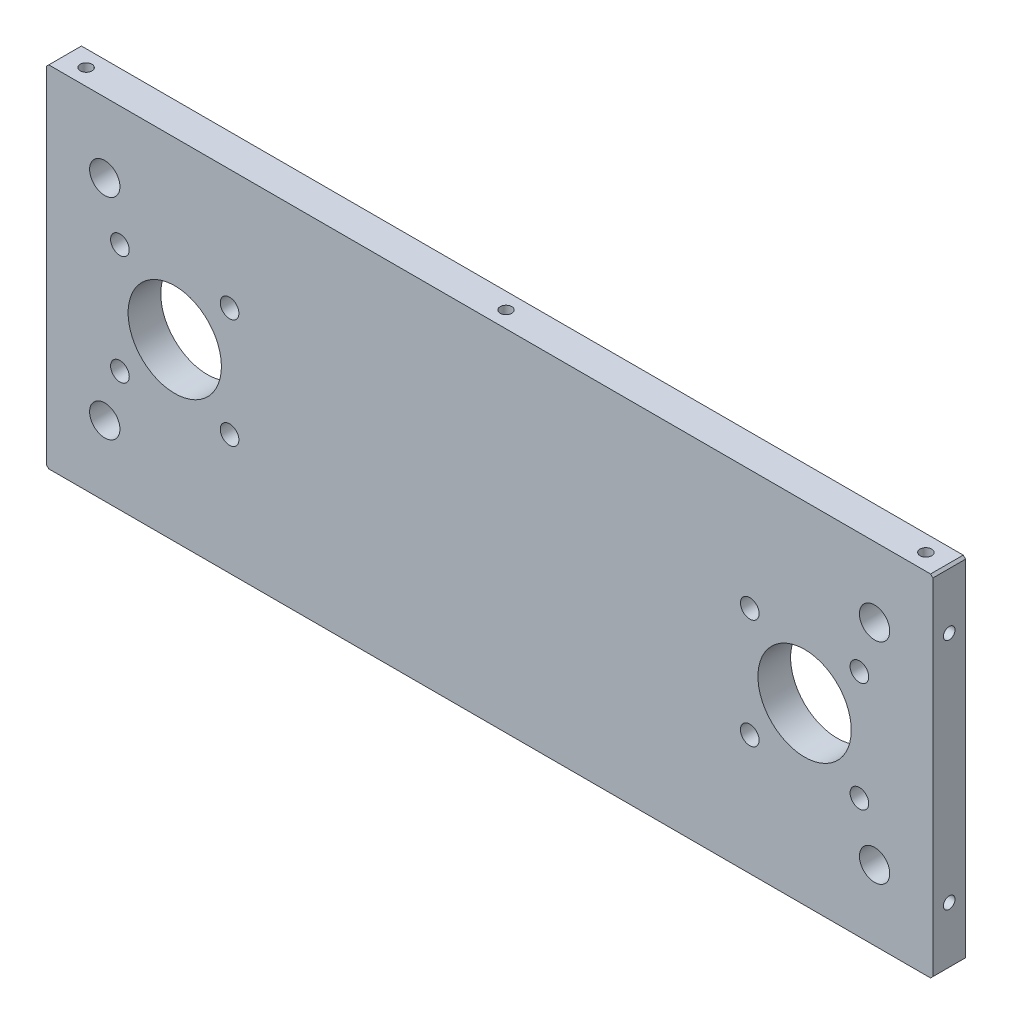
from build123d import *

# Parameters (mm, degrees)
SKETCH1_W                  = 380
SKETCH1_H                  = 150
BOSS_EXTRUDE1_DEPTH        = 14
CHAMFER1_SIZE              = 1
SKETCH2_R                  = 20
CUT_EXTRUDE1_DEPTH         = 409.773776067
F_8_0_8_DIAMETER_HOLE1_D   = 8
LPATTERN1_COUNT            = 2
LPATTERN1_PITCH            = 270
F_13_0_13_DIAMETER_HOLE1_D = 13
M6_TAPPED_HOLE1_D          = 5
M6_TAPPED_HOLE1_DEPTH      = 15
M6_TAPPED_HOLE1_TIP        = 1.502151548
M6_TAPPED_HOLE2_D          = 5
M6_TAPPED_HOLE2_DEPTH      = 15
M6_TAPPED_HOLE2_TIP        = 1.502151548
M6_TAPPED_HOLE3_D          = 5
M6_TAPPED_HOLE3_DEPTH      = 15
M6_TAPPED_HOLE3_TIP        = 1.502151548
M6_TAPPED_HOLE4_D          = 5
M6_TAPPED_HOLE4_DEPTH      = 15
M6_TAPPED_HOLE4_TIP        = 1.502151548


with BuildPart() as part:
    # Sketch1 → Boss-Extrude1 (new body)
    with BuildSketch(Plane.XY):
        with Locations((190, 75)):
            Rectangle(SKETCH1_W, SKETCH1_H)
    extrude(amount=BOSS_EXTRUDE1_DEPTH)

    # Chamfer1
    chamfer1_edges = [part.edges().sort_by_distance(p)[0] for p in [
        (0, 150, 7),
        (380, 150, 7),
        (380, 0, 7),
        (0, 0, 7),
    ]]
    chamfer(chamfer1_edges, length=CHAMFER1_SIZE)

    # Sketch2 → Cut-Extrude1 (cut, through all)
    with BuildSketch(Plane.XY.offset(14)):
        with Locations((55, 75)):
            Circle(SKETCH2_R)
        with Locations((325, 75)):
            Circle(SKETCH2_R)
    extrude(amount=-CUT_EXTRUDE1_DEPTH, mode=Mode.SUBTRACT)

    # Ø8.0 (8) Diameter Hole1 (through all)
    with Locations(Plane(origin=(31.5, 98.5, 14), x_dir=(1, 0, 0), z_dir=(0, 0, 1))):
        with Locations((0, 0), (47, 0), (47, -47), (0, -47)):
            f_8_0_8_diameter_hole1 = Hole(F_8_0_8_DIAMETER_HOLE1_D / 2)

    # LPattern1: Ø8.0 (8) Diameter Hole1 ×2
    with Locations(*[(i * LPATTERN1_PITCH, 0, 0) for i in range(1, LPATTERN1_COUNT)]):
        add(f_8_0_8_diameter_hole1, mode=Mode.SUBTRACT)

    # Ø13.0 (13) Diameter Hole1 (through all)
    with Locations(Plane(origin=(355, 120, 0), x_dir=(-1, 0, 0), z_dir=(0, 0, -1))):
        with Locations((0, 0), (0, -90), (330, -90), (330, 0)):
            Hole(F_13_0_13_DIAMETER_HOLE1_D / 2)

    # M6 Tapped Hole1
    with Locations(Plane(origin=(0, 0, 0), x_dir=(-1, 0, 0), z_dir=(0, -1, 0))):
        with Locations((-370, -7), (-190, -7), (-10, -7)):
            Hole(M6_TAPPED_HOLE1_D / 2, depth=M6_TAPPED_HOLE1_DEPTH)
            with Locations((0, 0, -(M6_TAPPED_HOLE1_DEPTH + M6_TAPPED_HOLE1_TIP / 2))):  # 118° drill point
                Cone(0, M6_TAPPED_HOLE1_D / 2, M6_TAPPED_HOLE1_TIP, mode=Mode.SUBTRACT)

    # M6 Tapped Hole2
    with Locations(Plane(origin=(0, 150, 0), x_dir=(1, 0, 0), z_dir=(0, 1, 0))):
        with Locations((370, -7), (190, -7), (10, -7)):
            Hole(M6_TAPPED_HOLE2_D / 2, depth=M6_TAPPED_HOLE2_DEPTH)
            with Locations((0, 0, -(M6_TAPPED_HOLE2_DEPTH + M6_TAPPED_HOLE2_TIP / 2))):  # 118° drill point
                Cone(0, M6_TAPPED_HOLE2_D / 2, M6_TAPPED_HOLE2_TIP, mode=Mode.SUBTRACT)

    # M6 Tapped Hole3
    with Locations(Plane(origin=(380, 0, 0), x_dir=(0, 0, -1), z_dir=(1, 0, 0))):
        with Locations((-7, 125), (-7, 25)):
            Hole(M6_TAPPED_HOLE3_D / 2, depth=M6_TAPPED_HOLE3_DEPTH)
            with Locations((0, 0, -(M6_TAPPED_HOLE3_DEPTH + M6_TAPPED_HOLE3_TIP / 2))):  # 118° drill point
                Cone(0, M6_TAPPED_HOLE3_D / 2, M6_TAPPED_HOLE3_TIP, mode=Mode.SUBTRACT)

    # M6 Tapped Hole4
    with Locations(Plane.ZY):
        with Locations((7, 25), (7, 125)):
            Hole(M6_TAPPED_HOLE4_D / 2, depth=M6_TAPPED_HOLE4_DEPTH)
            with Locations((0, 0, -(M6_TAPPED_HOLE4_DEPTH + M6_TAPPED_HOLE4_TIP / 2))):  # 118° drill point
                Cone(0, M6_TAPPED_HOLE4_D / 2, M6_TAPPED_HOLE4_TIP, mode=Mode.SUBTRACT)


solid = part.part
